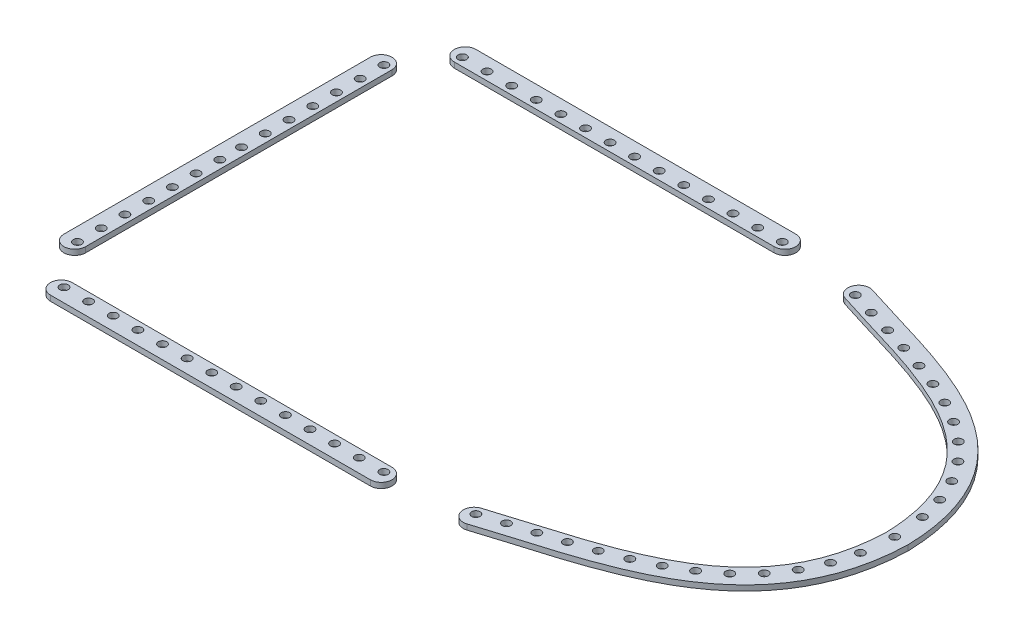
SolidWorks part; units mm, degrees
material "Thornel Mat VMA"
ref_plane "前视基准面" through (0, 0, 0) normal (0, 0, 1) x (1, 0, 0)
ref_plane "上视基准面" through (0, 0, 0) normal (0, 1, 0) x (1, 0, 0)
ref_plane "右视基准面" through (0, 0, 0) normal (1, 0, 0) x (0, 0, -1)
other "Configuration Table"
sketch "草图1" plane through (0, 0, 0) normal (0, 1, 0) x (1, 0, 0)
  line L0 (0, 0) -> (116, 0) construction
  line L1 (0, 0) -> (184.9718, 184.9718) construction
  line L2 (116, 52) -> (66.5454, 70) construction
  line L3 (66.5454, 70) -> (0, 70) construction
  line L4 (0, 70) -> (0, 0) construction
  line L5 (-73.5, 73.5) -> (56.5294, 73.5) construction
  line L6 (0, 0) -> (-151.1154, 151.1154) construction
  line L7 (56.5294, 73.5) -> (-61.5, 73.5) construction
  line L8 (-73.5, 56.5294) -> (-73.5, -56.5294) construction
  line L9 (56.5294, -70.5) -> (-61.5, -70.5)
  line L10 (-78.5, 56.5294) -> (-78.5, -56.5294)
  line L11 (56.5294, 78.5) -> (-61.5, 78.5)
  line L12 (56.5294, -78.5) -> (-61.5, -78.5)
  line L13 (56.5294, 70.5) -> (-61.5, 70.5)
  line L14 (-70.5, 56.5294) -> (-70.5, -56.5294)
  line L15 (86.9706, 70) -> (95.5567, 67.3021) construction
  line L16 (-2.4853, 128.6991) -> (-2.4853, 73.5) construction
  line L17 (95.5567, 67.3021) -> (104.1749, 64.7086) construction
  line L18 (104.1749, 64.7086) -> (112.7735, 62.0508) construction
  line L19 (112.7735, 62.0508) -> (121.3011, 59.1732) construction
  line L20 (121.3011, 59.1732) -> (129.6919, 55.9184) construction
  line L21 (129.6919, 55.9184) -> (137.8499, 52.1175) construction
  line L22 (137.8499, 52.1175) -> (145.6287, 47.5908) construction
  line L23 (145.6287, 47.5908) -> (152.8111, 42.1674) construction
  line L24 (152.8111, 42.1674) -> (159.1093, 35.7384) construction
  line L25 (159.1093, 35.7384) -> (164.2223, 28.3319) construction
  line L26 (164.2223, 28.3319) -> (167.9529, 20.1414) construction
  line L27 (167.9529, 20.1414) -> (170.2921, 11.4508) construction
  circle A0 centre (116, 0) radius 52 construction
  circle A1 centre (-73.5, -56.5294) radius 1.55
  circle A2 centre (-73.5, -47.7745) radius 1.55
  circle A3 centre (-73.5, -39.0196) radius 1.55
  circle A4 centre (-73.5, -30.2647) radius 1.55
  circle A5 centre (-73.5, -21.5098) radius 1.55
  circle A6 centre (-73.5, -12.7549) radius 1.55
  circle A7 centre (-73.5, -4) radius 1.55
  circle A8 centre (-73.5, 4) radius 1.55
  circle A9 centre (-73.5, 12.7549) radius 1.55
  circle A10 centre (-73.5, 21.5098) radius 1.55
  circle A11 centre (-73.5, 30.2647) radius 1.55
  circle A12 centre (-73.5, 39.0196) radius 1.55
  circle A13 centre (-73.5, 47.7745) radius 1.55
  circle A14 centre (-73.5, 56.5294) radius 1.55
  arc A15 (-78.5, 56.5294) -> (-70.5, 56.5294) centre (-74.5, 56.5294) cw
  arc A16 (-78.5, -56.5294) -> (-70.5, -56.5294) centre (-74.5, -56.5294) ccw
  circle A17 centre (-61.5, 73.5) radius 1.55
  circle A18 centre (-52.4142, 73.5) radius 1.55
  circle A19 centre (-43.3284, 73.5) radius 1.55
  circle A20 centre (-34.2426, 73.5) radius 1.55
  circle A21 centre (-25.1569, 73.5) radius 1.55
  circle A22 centre (-16.0711, 73.5) radius 1.55
  circle A23 centre (-6.9853, 73.5) radius 1.55
  circle A24 centre (2.0147, 73.5) radius 1.55
  circle A25 centre (11.1005, 73.5) radius 1.55
  circle A26 centre (20.1863, 73.5) radius 1.55
  circle A27 centre (29.2721, 73.5) radius 1.55
  circle A28 centre (38.3579, 73.5) radius 1.55
  circle A29 centre (47.4437, 73.5) radius 1.55
  circle A30 centre (56.5294, 73.5) radius 1.55
  arc A31 (-61.5, 78.5) -> (-61.5, 70.5) centre (-61.5, 74.5) ccw
  arc A32 (56.5294, 78.5) -> (56.5294, 70.5) centre (56.5294, 74.5) cw
  arc A33 (56.5294, -78.5) -> (56.5294, -70.5) centre (56.5294, -74.5) ccw
  arc A34 (-61.5, -78.5) -> (-61.5, -70.5) centre (-61.5, -74.5) cw
  circle A35 centre (56.5294, -73.5) radius 1.55
  circle A36 centre (47.4437, -73.5) radius 1.55
  circle A37 centre (38.3579, -73.5) radius 1.55
  circle A38 centre (29.2721, -73.5) radius 1.55
  circle A39 centre (20.1863, -73.5) radius 1.55
  circle A40 centre (11.1005, -73.5) radius 1.55
  circle A41 centre (2.0147, -73.5) radius 1.55
  circle A42 centre (-6.9853, -73.5) radius 1.55
  circle A43 centre (-16.0711, -73.5) radius 1.55
  circle A44 centre (-25.1569, -73.5) radius 1.55
  circle A45 centre (-34.2426, -73.5) radius 1.55
  circle A46 centre (-43.3284, -73.5) radius 1.55
  circle A47 centre (-52.4142, -73.5) radius 1.55
  circle A48 centre (-61.5, -73.5) radius 1.55
  circle A49 centre (86.9706, 70) radius 1.55
  arc A50 (86.0326, 67.1504) -> (88.5338, 74.7493) centre (87.2832, 70.9499) cw
  circle A51 centre (95.5567, 67.3021) radius 1.55
  circle A52 centre (104.1749, 64.7086) radius 1.55
  circle A53 centre (112.7735, 62.0508) radius 1.55
  circle A54 centre (121.3011, 59.1732) radius 1.55
  circle A55 centre (129.6919, 55.9184) radius 1.55
  circle A56 centre (137.8499, 52.1175) radius 1.55
  circle A57 centre (145.6287, 47.5908) radius 1.55
  circle A59 centre (152.8111, 42.1674) radius 1.55
  circle A60 centre (159.1093, 35.7384) radius 1.55
  circle A61 centre (164.2223, 28.3319) radius 1.55
  circle A62 centre (167.9529, 20.1414) radius 1.55
  circle A63 centre (170.2921, 11.4508) radius 1.55
  circle A64 centre (171.5, 0) radius 1.55
  arc A65 (86.0326, -67.1504) -> (88.5338, -74.7493) centre (87.2832, -70.9499) ccw
  circle A66 centre (170.2921, -11.4508) radius 1.55
  circle A67 centre (167.9529, -20.1414) radius 1.55
  circle A68 centre (164.2223, -28.3319) radius 1.55
  circle A69 centre (159.1093, -35.7384) radius 1.55
  circle A70 centre (152.8111, -42.1674) radius 1.55
  circle A71 centre (145.6287, -47.5908) radius 1.55
  circle A72 centre (137.8499, -52.1175) radius 1.55
  circle A73 centre (129.6919, -55.9184) radius 1.55
  circle A74 centre (121.3011, -59.1732) radius 1.55
  circle A75 centre (112.7735, -62.0508) radius 1.55
  circle A76 centre (104.1749, -64.7086) radius 1.55
  circle A77 centre (95.5567, -67.3021) radius 1.55
  circle A78 centre (86.9706, -70) radius 1.55
  spline S0 degree 3 poles (171.5, 0) (170.0053, 51.3068) (122.3458, 58.3562) (86.9706, 70) knots 0 0 0 0 1 1 1 1 construction
  spline S1 degree 3 poles (171.5, 0) (170.0053, -51.3068) (122.3458, -58.3562) (86.9706, -70) knots 0 0 0 0 1 1 1 1 construction
  spline S2 degree 1 poles (176.5021, 0) (88.5338, -74.7493) knots 0 0 1 1 construction
  spline S3 degree 1 poles (176.5021, 0) (88.5338, 74.7493) knots 0 0 1 1 construction
  spline S4 degree 3 poles (88.5338, -74.7493) (89.6307, -74.3883) (91.8125, -73.6867) (96.3247, -72.2852) (102.1172, -70.548) (109.2519, -68.4076) (118.8823, -65.3862) (130.931, -61.1065) (144.7335, -54.5247) (155.1079, -47.2387) (162.3016, -39.9713) (167.0143, -33.7318) (170.9154, -26.655) (173.3921, -20.0384) (174.8626, -14.3028) (175.7011, -9.777) (176.1716, -5.813) (176.4088, -2.5281) (176.4777, -0.8392) (176.5021, 0) knots -0.000946 -0.000946 -0.000946 -0.000946 0.030334 0.061613 0.124172 0.186731 0.249291 0.374409 0.499527 0.624645 0.687204 0.749764 0.812323 0.874882 0.906161 0.937441 0.96872 0.98436 1 1 1 1
  spline S5 degree 3 poles (176.5021, 0) (176.4777, 0.8392) (176.4088, 2.5281) (176.1716, 5.813) (175.7011, 9.777) (174.8626, 14.3028) (173.3921, 20.0384) (170.9154, 26.655) (167.0143, 33.7318) (162.3016, 39.9713) (155.1079, 47.2387) (144.7335, 54.5247) (130.931, 61.1065) (118.8823, 65.3862) (109.2519, 68.4076) (102.1172, 70.548) (96.3247, 72.2852) (91.8125, 73.6867) (89.6307, 74.3883) (88.5338, 74.7493) knots -0.000946 -0.000946 -0.000946 -0.000946 0.014694 0.030334 0.061613 0.092893 0.124172 0.186731 0.249291 0.31185 0.374409 0.499527 0.624645 0.749764 0.812323 0.874882 0.937441 0.96872 1 1 1 1
  spline S6 degree 1 poles (168.4987, 0) (86.0326, 67.1504) knots 0 0 1 1 construction
  spline S7 degree 1 poles (168.4987, 0) (86.0326, -67.1504) knots 0 0 1 1 construction
  spline S8 degree 3 poles (86.0326, 67.1504) (87.1578, 66.78) (89.4033, 66.058) (93.9888, 64.6338) (99.8137, 62.8868) (106.8877, 60.7646) (116.313, 57.8081) (127.8712, 53.6996) (140.6897, 47.578) (149.9312, 41.0776) (156.169, 34.7945) (160.2101, 29.4683) (163.5545, 23.4431) (165.7055, 17.7576) (167.0042, 12.759) (167.7555, 8.7744) (168.1862, 5.242) (168.4069, 2.2969) (168.4757, 0.7607) (168.4987, 0) knots 0.000589 0.000589 0.000589 0.000589 0.031821 0.063052 0.125515 0.187979 0.250442 0.375368 0.500295 0.625221 0.687684 0.750147 0.81261 0.875074 0.906305 0.937537 0.968768 0.984384 1 1 1 1
  spline S9 degree 3 poles (168.4987, 0) (168.4757, -0.7607) (168.4069, -2.2969) (168.1862, -5.242) (167.7555, -8.7744) (167.0042, -12.759) (165.7055, -17.7576) (163.5545, -23.4431) (160.2101, -29.4683) (156.169, -34.7945) (149.9312, -41.0776) (140.6897, -47.578) (127.8712, -53.6996) (116.313, -57.8081) (106.8877, -60.7646) (99.8137, -62.8868) (93.9888, -64.6338) (89.4033, -66.058) (87.1578, -66.78) (86.0326, -67.1504) knots 0.000589 0.000589 0.000589 0.000589 0.016205 0.031821 0.063052 0.094284 0.125515 0.187979 0.250442 0.312905 0.375368 0.500295 0.625221 0.750147 0.81261 0.875074 0.937537 0.968768 1 1 1 1
  point P34 (-73.5, 0)
  point P185 (85.7898, -67.2421)
  point P186 (88.9384, -74.5)
  point P187 (88.9384, 74.5965)
  point P188 (85.7898, 67.2421)
  dimension "D2" = 104
  dimension "D20" = 3.1
  dimension "D21" = 7
  dimension "D22" = 8
  dimension "D23" = 4
  dimension "4" = 4
  dimension "D25" = 3.1
  dimension "D27" = 9
  dimension "D28" = 4
  dimension "D29" = 4
  dimension "D30" = 3.1
  dimension "D31" = 4
  dimension "D32" = 9
  dimension "D1" = 116
  dimension "D3" = 45
  dimension "D4" = 70
  dimension "D5" = 20
  dimension "D6" = 12
  dimension "D7" = 55.5
  dimension "D8" = 3.5
  dimension "D9" = 189.5
  dimension "D10" = 12
  dimension "D11" = 12
  dimension "D12" = 12
  dimension "D13" = 61
  dimension "D14" = 116
  dimension "D15" = 48
  dimension "D16" = 145
  dimension "D17" = 5
  dimension "D18" = 3
  dimension "D19" = 3
  dimension "D24" = 8
  dimension "D26" = 7
extrude "凸台-拉伸1" add sketch "草图1" along normal blind 2
